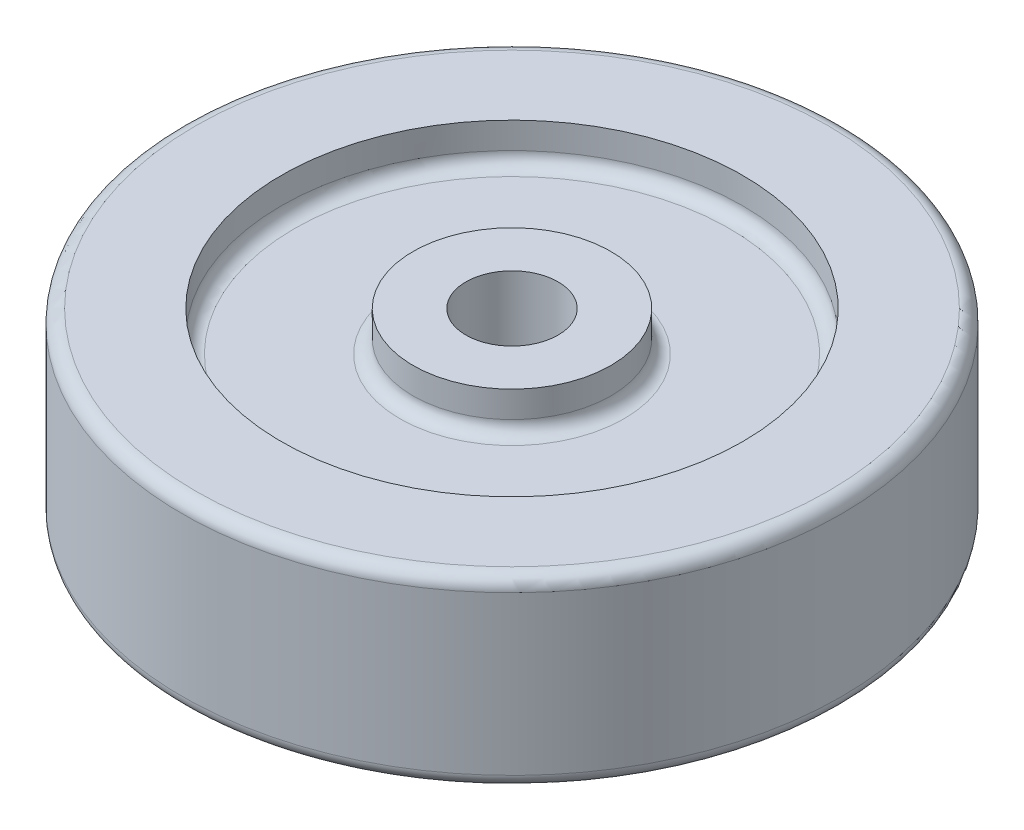
SolidWorks part; units mm, degrees
ref_plane "Front Plane" through (0, 0, 0) normal (0, 0, 1) x (1, 0, 0)
ref_plane "Top Plane" through (0, 0, 0) normal (0, 1, 0) x (1, 0, 0)
ref_plane "Right Plane" through (0, 0, 0) normal (1, 0, 0) x (0, 0, -1)
sketch "Sketch1" plane through (0, 0, 0) normal (0, 0, 1) x (1, 0, 0)
  line L0 (0, -499.995) -> (0, 24499.753) construction
  line L1 (15, 8) -> (35, 8)
  line L2 (7, 14) -> (15, 14)
  line L3 (7, 14) -> (7, -14)
  line L4 (7, -14) -> (15, -14)
  line L5 (15, 14) -> (15, 8)
  line L6 (35, 8) -> (35, 14)
  line L7 (35, 14) -> (50, 14)
  line L8 (50, 14) -> (50, -14)
  line L9 (50, -14) -> (35, -14)
  line L10 (35, -14) -> (35, -8)
  line L11 (35, -8) -> (15, -8)
  line L12 (15, -8) -> (15, -14)
  dimension "D1" = 7
  dimension "D2" = 15
  dimension "D3" = 14
  dimension "D4" = 6
  dimension "D5" = 28
  dimension "D6" = 14
  dimension "D7" = 35
  dimension "D8" = 16
  dimension "D9" = 50
revolve "Revolve1" add sketch "Sketch1" angle 360 about L0
fillet "Fillet2" radius 2 3 edges at (50, 14, 0) (35, 8, 0) (15, 8, 0)
fillet "Fillet4" radius 2 3 edges at (15, -8, 0) (35, -8, 0) (50, -14, 0)
